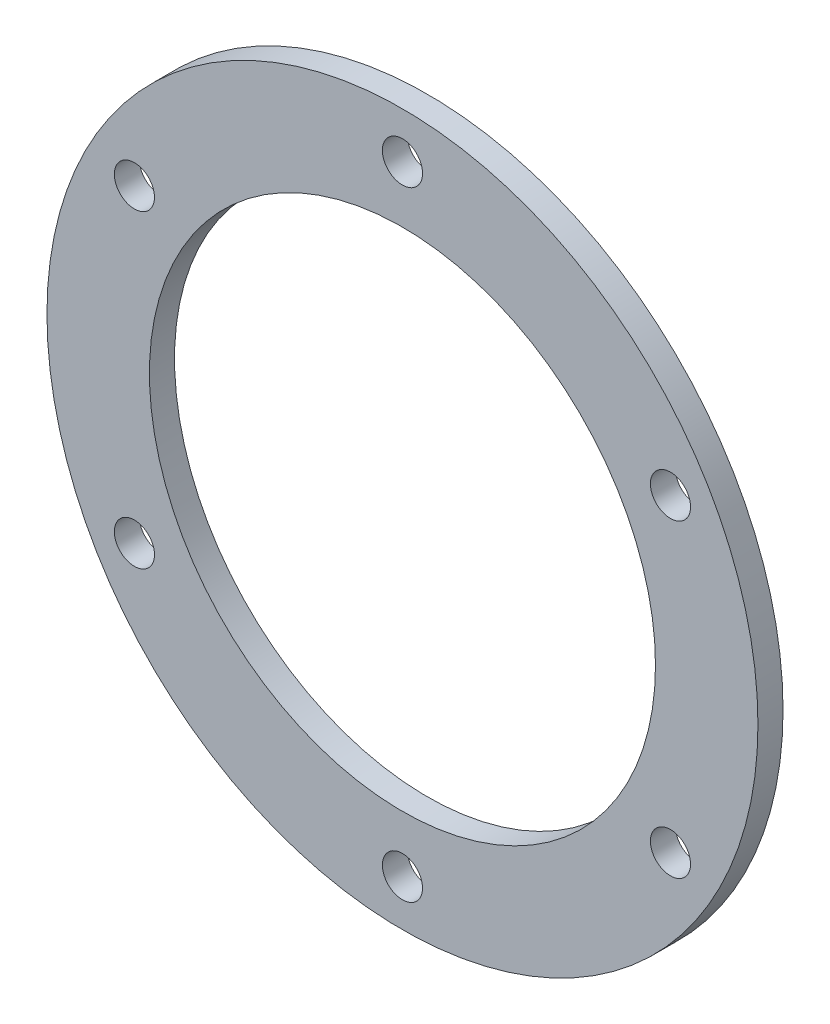
from build123d import *

# Parameters (mm, degrees)
SKETCH1_R           = 42.5
SKETCH1_R_2         = 30.25
BOSS_EXTRUDE1_DEPTH = 3
SKETCH2_R           = 2.4
CUT_EXTRUDE1_DEPTH  = 3


with BuildPart() as part:
    # Sketch1 → Boss-Extrude1 (new body)
    with BuildSketch(Plane.XY):
        Circle(SKETCH1_R)
        Circle(SKETCH1_R_2, mode=Mode.SUBTRACT)
    extrude(amount=BOSS_EXTRUDE1_DEPTH)

    # Sketch2 → Cut-Extrude1 (cut)
    with BuildSketch(Plane.XY.offset(3)):
        with Locations((0, 37)):
            Circle(SKETCH2_R)
        with Locations((32.04293994, 18.5)):
            Circle(SKETCH2_R)
        with Locations((32.04293994, -18.5)):
            Circle(SKETCH2_R)
        with Locations((0, -37)):
            Circle(SKETCH2_R)
        with Locations((-32.04293994, -18.5)):
            Circle(SKETCH2_R)
        with Locations((-32.04293994, 18.5)):
            Circle(SKETCH2_R)
    extrude(amount=-CUT_EXTRUDE1_DEPTH, mode=Mode.SUBTRACT)


solid = part.part
